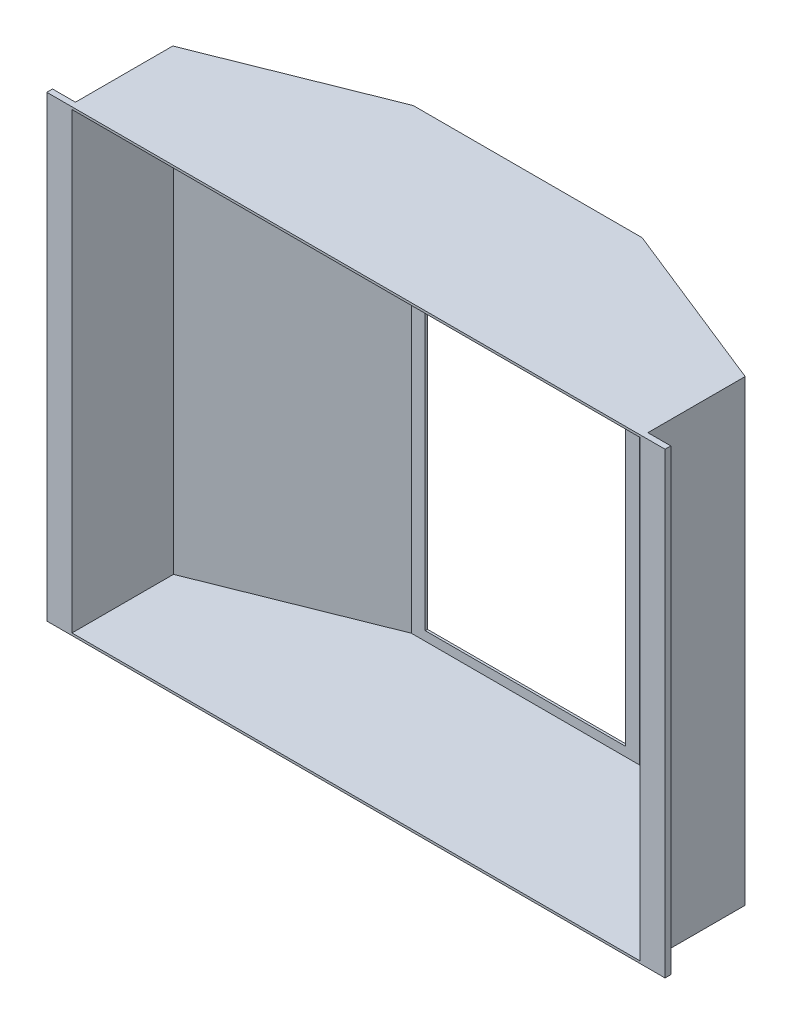
SolidWorks part; units mm, degrees
ref_plane "前视基准面" through (0, 0, 0) normal (0, 0, 1) x (1, 0, 0)
ref_plane "上视基准面" through (0, 0, 0) normal (0, 1, 0) x (1, 0, 0)
ref_plane "右视基准面" through (0, 0, 0) normal (1, 0, 0) x (0, 0, -1)
sketch "草图1" plane through (0, 0, 0) normal (0, 0, 1) x (1, 0, 0)
  line L1 (-250, -200) -> (250, -200)
  line L2 (-250, -200) -> (-250, 200)
  line L3 (-250, 200) -> (250, 200)
  line L4 (250, -200) -> (250, 200)
  line L5 (-250, -200) -> (250, 200) construction
  line L6 (-250, 200) -> (250, -200) construction
  point P0 (0, 0)
  dimension "D1" = 500
  dimension "D2" = 400
extrude "凸台-拉伸1" add sketch "草图1" along normal blind 150
sketch "草图3" plane through (0, -200, 0) normal (0, -1, 0) x (1, 0, 0)
  line L0 (-100, 0) -> (-250, 60)
  line L1 (-250, 0) -> (250, 0) construction
  line L2 (-250, 150) -> (-250, 0) construction
  line L3 (-250, 60) -> (-250, 0)
  line L4 (-250, 0) -> (-100, 0)
  line L5 (250, 60) -> (100, 0)
  line L6 (250, 150) -> (250, 0) construction
  line L7 (100, 0) -> (250, 0)
  line L8 (250, 0) -> (250, 60)
  dimension "D1" = 60
  dimension "D2" = 150
extrude "切除-拉伸1" cut sketch "草图3" against normal through all
shell "抽壳1" thickness 2
sketch "草图2" plane through (0, 0, 150) normal (0, 0, 1) x (1, 0, 0)
  line L0 (-250, -200) -> (250, -200) construction
  line L1 (-250, 200) -> (-270, 200)
  line L2 (-250, 200) -> (-250, -200)
  line L3 (-250, -200) -> (-270, -200)
  line L4 (-270, 200) -> (-270, -200)
  line L6 (250, 200) -> (270, 200)
  line L7 (250, 200) -> (250, -200)
  line L8 (250, -200) -> (270, -200)
  line L9 (270, 200) -> (270, -200)
  dimension "D1" = 20
extrude "凸台-拉伸2" add sketch "草图2" against normal blind 5
sketch "草图4" plane through (0, 0, 2) normal (0, 0, 1) x (1, 0, 0)
  line L1 (-87.5, -190) -> (87.5, -190)
  line L2 (-87.5, -190) -> (-87.5, 190)
  line L3 (-87.5, 190) -> (87.5, 190)
  line L4 (87.5, -190) -> (87.5, 190)
  line L5 (-87.5, -190) -> (87.5, 190) construction
  line L6 (-87.5, 190) -> (87.5, -190) construction
  point P0 (0, 0)
  dimension "D1" = 175
  dimension "D2" = 380
extrude "切除-拉伸2" cut sketch "草图4" against normal through all
